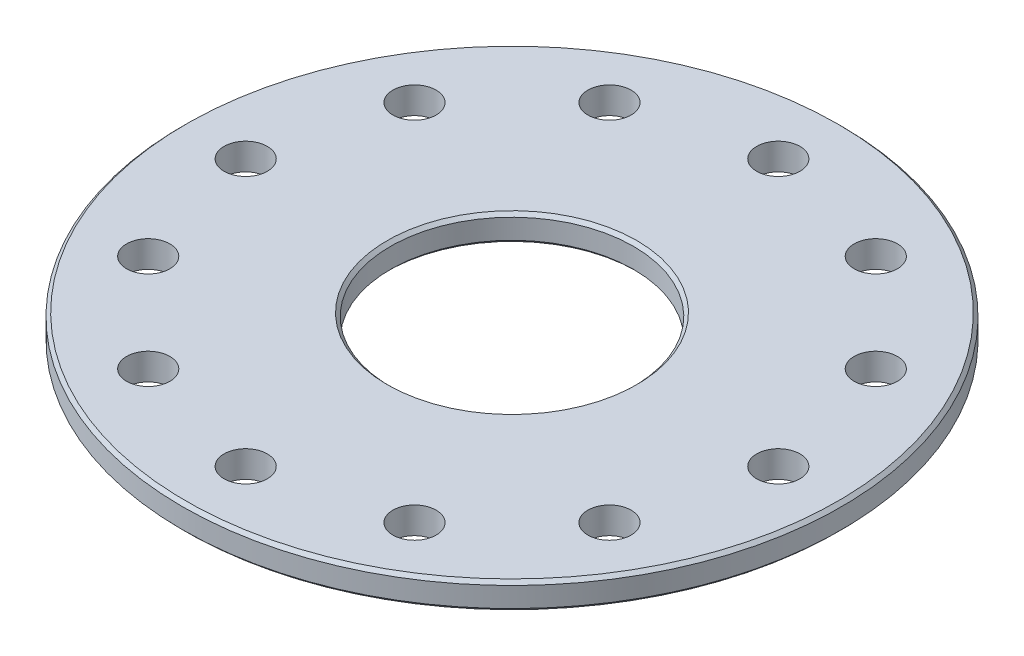
SolidWorks part; units mm, degrees
material "Q235A"
ref_plane "前视基准面" through (0, 0, 0) normal (0, 0, 1) x (1, 0, 0)
ref_plane "上视基准面" through (0, 0, 0) normal (0, 1, 0) x (1, 0, 0)
ref_plane "右视基准面" through (0, 0, 0) normal (1, 0, 0) x (0, 0, -1)
ref_plane "基准面1" through (0, 87, 0) normal (0, 1, 0) x (1, 0, 0)
sketch "草图1" plane through (0, 87, 0) normal (0, 1, 0) x (1, 0, 0)
  circle A0 centre (0, 0) radius 99
  circle A1 centre (-80, 0) radius 6.5
  circle A2 centre (40, 69.282) radius 6.5
  circle A3 centre (-69.282, 40) radius 6.5
  circle A4 centre (-69.282, -40) radius 6.5
  circle A5 centre (0, 80) radius 6.5
  circle A6 centre (69.282, -40) radius 6.5
  circle A7 centre (-40, 69.282) radius 6.5
  circle A8 centre (0, -80) radius 6.5
  circle A9 centre (40, -69.282) radius 6.5
  circle A10 centre (69.282, 40) radius 6.5
  circle A11 centre (-40, -69.282) radius 6.5
  circle A12 centre (80, 0) radius 6.5
  circle A13 centre (0, 0) radius 36.5
  dimension "D1" = 13
  dimension "D2" = 73
  dimension "D3" = 198
  dimension "D17" = 73
  dimension "D4" = 40
  dimension "D5" = 69.282
  dimension "D6" = 80
  dimension "D7" = 40
  dimension "D8" = 69.282
  dimension "D9" = 80
  dimension "D10" = 40
  dimension "D11" = 69.282
  dimension "D12" = 80
  dimension "D13" = 40
  dimension "D14" = 69.282
  dimension "D15" = 80
extrude "凸台-拉伸1" add sketch "草图1" against normal blind 8
chamfer "倒角1" distance 1 angle 45 4 edges at (0, 87, -99) (0, 79, -99) (0, 87, -36.5) (0, 79, -36.5)
